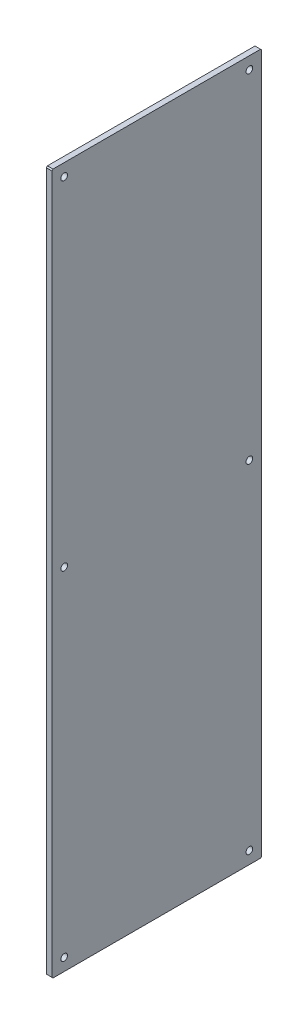
from build123d import *

# Parameters (mm, degrees)
SKETCH_1_W          = 188
SKETCH_1_H          = 628
EXTRUDE_1_DEPTH     = 5
CHAMFER_1_SIZE      = 1
SKETCH_2_R          = 3
CUT_EXTRUDE_1_DEPTH = 328.806345271


with BuildPart() as part:
    # 草图1 → 凸台-拉伸1 (new body)
    with BuildSketch(Plane(origin=(0, 0, 0), x_dir=(0, 0, -1), z_dir=(1, 0, 0))):
        Rectangle(SKETCH_1_W, SKETCH_1_H)
    extrude(amount=EXTRUDE_1_DEPTH)

    # 倒角1
    chamfer_1_edges = [part.edges().sort_by_distance(p)[0] for p in [
        (2.5, 314, 94),
        (2.5, 314, -94),
        (2.5, -314, -94),
        (2.5, -314, 94),
    ]]
    chamfer(chamfer_1_edges, length=CHAMFER_1_SIZE)

    # 草图2 → 切除-拉伸1 (cut, through all)
    with BuildSketch(Plane.ZY):
        with Locations((-83, 303)):
            Circle(SKETCH_2_R)
        with Locations(Location((-83, -303, 0), (0, 0, 180))):
            Circle(SKETCH_2_R)
        with Locations((83, -303)):
            Circle(SKETCH_2_R)
        with Locations(Location((83, 303, 0), (0, 0, 180))):
            Circle(SKETCH_2_R)
        with Locations((83, 0)):
            Circle(SKETCH_2_R)
        with Locations((-83, 0)):
            Circle(SKETCH_2_R)
    extrude(amount=-CUT_EXTRUDE_1_DEPTH, mode=Mode.SUBTRACT)


solid = part.part
